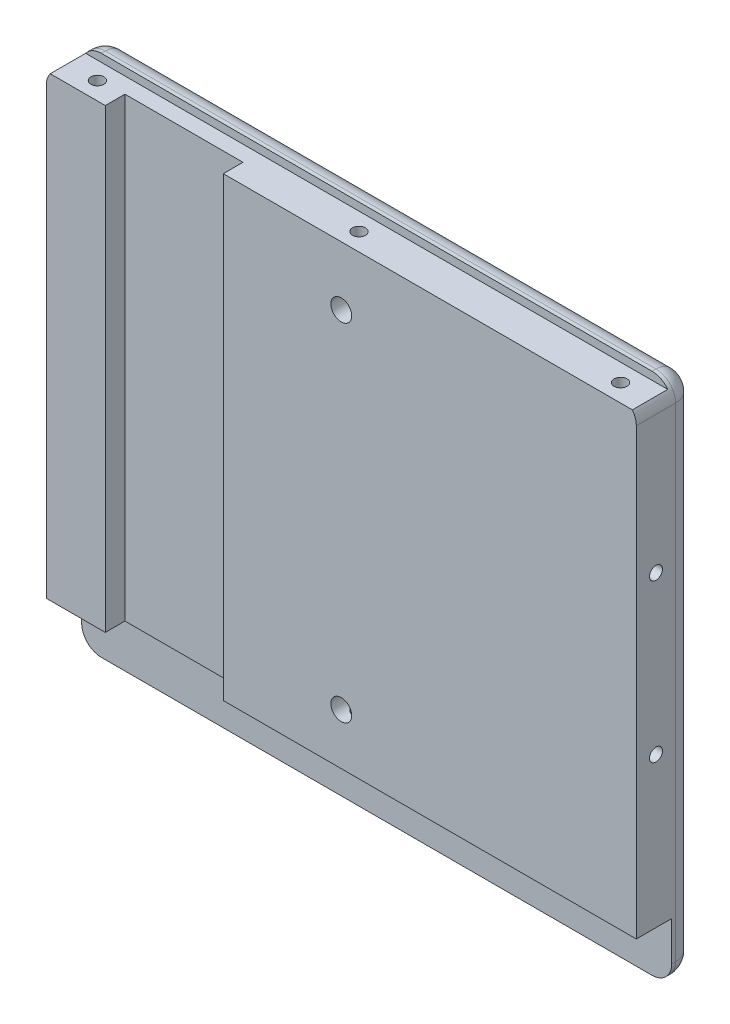
from build123d import *

# Parameters (mm, degrees)
SKETCH_1_W                  = 150
SKETCH_1_H                  = 133
EXTRUDE_1_DEPTH             = 15
SKETCH_2_W                  = 32.584056601
SKETCH_2_H                  = 28.363937547
CUT_EXTRUDE_1_DEPTH         = 165.764225486
FILLET_8_R                  = 5
HOLE_WIZARD_1_D             = 5.3
HOLE_WIZARD_1_CBORE_D       = 10
HOLE_WIZARD_1_CBORE_DEPTH   = 5.7
HOLE_WIZARD_M4_3_D          = 3.3
HOLE_WIZARD_M4_3_DEPTH      = 15.5
HOLE_WIZARD_M4_3_TIP        = 0.991420021
SKETCH_20_W                 = 431.741055117
SKETCH_20_H                 = 139.105675049
CUT_EXTRUDE_5_DEPTH         = 15
SKETCH_24_W                 = 30
SKETCH_24_H                 = 177.502907688
CUT_EXTRUDE_6_DEPTH         = 5
HOLE_WIZARD_M4_2_D          = 3.3
HOLE_WIZARD_M4_2_DEPTH      = 11.5
HOLE_WIZARD_M4_2_TIP        = 0.991420021
HOLE_WIZARD_M4_1_AT_2_COUNT = 2
HOLE_WIZARD_M4_1_AT_2_PITCH = 40


with BuildPart() as part:
    # 草图1 → 凸台-拉伸1 (new body)
    with BuildSketch(Plane.XY):
        Rectangle(SKETCH_1_W, SKETCH_1_H)
    extrude(amount=EXTRUDE_1_DEPTH)

    # 草图2 → 切除-拉伸1 (cut, through all)
    with BuildSketch(Plane(origin=(75, 0, 0), x_dir=(0, 0, -1), z_dir=(1, 0, 0))):
        with Locations((-22.292028301, 78.681968774)):
            Rectangle(SKETCH_2_W, SKETCH_2_H)
    extrude(amount=-CUT_EXTRUDE_1_DEPTH, mode=Mode.SUBTRACT)

    # 圆角8
    fillet_8_edges = [part.edges().sort_by_distance(p)[0] for p in [
        (75, 66.5, 3),
        (-75, 66.5, 3),
        (-75, -66.5, 7.5),
        (75, -66.5, 7.5),
        (0, -66.5, 0),
        (-75, 0, 0),
        (75, 0, 0),
        (0, 66.5, 0),
    ]]
    fillet(fillet_8_edges, radius=FILLET_8_R)

    # 打孔尺寸(%根据)开槽圆柱头螺钉的类型1 (through all)
    with Locations(Plane(origin=(0, 0, 0), x_dir=(-1, 0, 0), z_dir=(0, 0, -1))):
        with Locations((0, 49.5), (0, -38.5)):
            CounterBoreHole(HOLE_WIZARD_1_D / 2, HOLE_WIZARD_1_CBORE_D / 2, HOLE_WIZARD_1_CBORE_DEPTH)

    # M4 螺纹孔3
    with Locations(Plane(origin=(0, 64.5, 0), x_dir=(1, 0, 0), z_dir=(0, 1, 0))):
        with Locations((0, -10.5), (66.5, -10.5), (-66.5, -10.5)):
            Hole(HOLE_WIZARD_M4_3_D / 2, depth=HOLE_WIZARD_M4_3_DEPTH)
            with Locations((0, 0, -(HOLE_WIZARD_M4_3_DEPTH + HOLE_WIZARD_M4_3_TIP / 2))):  # 118° drill point
                Cone(0, HOLE_WIZARD_M4_3_D / 2, HOLE_WIZARD_M4_3_TIP, mode=Mode.SUBTRACT)

    # 草图20 → 切除-拉伸5 (cut)
    with BuildSketch(Plane.XZ.offset(66.5)):
        with Locations((-98.598792732, 75.552837525)):
            Rectangle(SKETCH_20_W, SKETCH_20_H)
    extrude(amount=-CUT_EXTRUDE_5_DEPTH, mode=Mode.SUBTRACT)

    # 草图24 → 切除-拉伸6 (cut)
    with BuildSketch(Plane.XY.offset(15)):
        with Locations((-45, -6.351602415)):
            Rectangle(SKETCH_24_W, SKETCH_24_H)
    extrude(amount=-CUT_EXTRUDE_6_DEPTH, mode=Mode.SUBTRACT)

    # M4 螺纹孔2
    with Locations(Plane(origin=(0, -51.5, 0), x_dir=(-1, 0, 0), z_dir=(0, -1, 0))):
        with Locations((66.5, -10.5), (0, -10.5), (-66.5, -10.5)):
            Hole(HOLE_WIZARD_M4_2_D / 2, depth=HOLE_WIZARD_M4_2_DEPTH)
            with Locations((0, 0, -(HOLE_WIZARD_M4_2_DEPTH + HOLE_WIZARD_M4_2_TIP / 2))):  # 118° drill point
                Cone(0, HOLE_WIZARD_M4_2_D / 2, HOLE_WIZARD_M4_2_TIP, mode=Mode.SUBTRACT)

    # 草图28 → M4 螺纹孔1 (revolve, cut)
    with BuildSketch(Plane(origin=(75, 26.61076125, 10), x_dir=(0, 0, -1), z_dir=(0, 1, 0))):
        Polygon((0, 0), (0, 12.991420021), (1.65, 12), (1.65, 0), align=None)
    hole_wizard_m4_1 = revolve(axis=Axis((81.35, 26.61076125, 10), (-1, 0, 0)), mode=Mode.SUBTRACT)

    # M4 螺纹孔1 at 2: M4 螺纹孔1 ×2
    with Locations(*[(0, -i * HOLE_WIZARD_M4_1_AT_2_PITCH, 0) for i in range(1, HOLE_WIZARD_M4_1_AT_2_COUNT)]):
        add(hole_wizard_m4_1, mode=Mode.SUBTRACT)

    # 镜向1: M4 螺纹孔1 across plane
    add(hole_wizard_m4_1.mirror(Plane(origin=(0, 0, 0), x_dir=(0, 0, 1), z_dir=(1, 0, 0))), mode=Mode.SUBTRACT)

    # 镜向1 copy 1 sketch → 镜向1 copy 1 (revolve, cut)
    with BuildSketch(Plane(origin=(-75, -13.38923875, 10), x_dir=(0, 0, -1), z_dir=(0, 1, 0))):
        Polygon((0, 0), (0, -12.991420021), (1.65, -12), (1.65, 0), align=None)
    revolve(axis=Axis((-81.35, -13.38923875, 10), (-1, 0, 0)), mode=Mode.SUBTRACT)


solid = part.part
